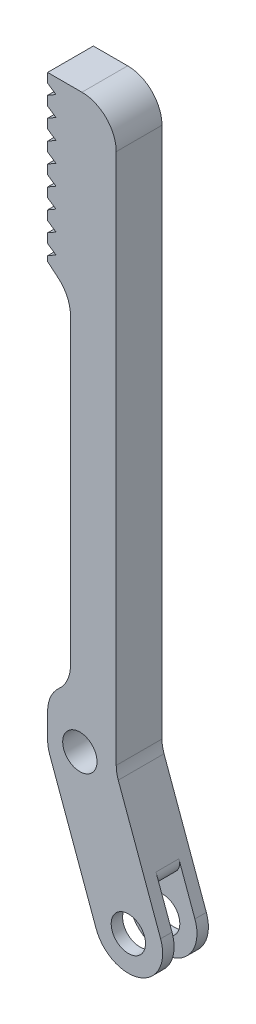
SolidWorks part; units mm, degrees
ref_plane "Front Plane" through (0, 0, 0) normal (0, 0, 1) x (1, 0, 0)
ref_plane "Top Plane" through (0, 0, 0) normal (0, 1, 0) x (1, 0, 0)
ref_plane "Right Plane" through (0, 0, 0) normal (1, 0, 0) x (0, 0, -1)
ref_plane "Plane1" through (0, 0, 20) normal (0, 0, 1) x (1, 0, 0)
sketch "Sketch1" plane through (0, 0, 20) normal (0, 0, 1) x (1, 0, 0)
  line L0 (-35.6011, 326.0365) -> (-35.6011, 70.7467)
  line L1 (-35.6011, 70.7467) -> (-14.3958, 12.4858)
  line L2 (13.7949, 22.7464) -> (-5.6011, 76.0365)
  line L3 (-5.6011, 76.0365) -> (-5.6011, 326.0365)
  line L4 (-5.6011, 326.0365) -> (-35.6011, 326.0365)
  arc A0 (-14.3958, 12.4858) -> (13.7949, 22.7464) centre (-0.3005, 17.6161) ccw
  dimension "D1" = 15
  dimension "D2" = 21.2052
  dimension "D3" = 30
  dimension "D4" = 35.3006
  dimension "D5" = 49.396
  dimension "D6" = 250
extrude "Boss-Extrude1" add sketch "Sketch1" against normal blind 20
sketch "Sketch2" plane through (19.4918, 7.0944, 0) normal (0.9397, 0.342, 0) x (0, 0, -1)
  line L0 (-15, -0.957) -> (-5, -0.957)
  line L1 (-5, -0.957) -> (-5, 32.1615)
  line L2 (-5, 32.1615) -> (-15, 32.1615)
  line L3 (-15, 32.1615) -> (-15, -0.957)
  dimension "D1" = 5
  dimension "D2" = 15
extrude "Cut-Extrude1" cut sketch "Sketch2" against normal up to next
sketch "Sketch3" plane through (0, 0, 0) normal (0, 0, -1) x (-1, 0, 0)
  line L0 (35.6011, 84.1696) -> (35.6011, 254.4275)
  line L1 (35.6011, 254.4275) -> (25.6011, 246.0365)
  line L2 (25.6011, 246.0365) -> (25.6011, 106.5303)
  line L3 (5.6011, 76.0365) -> (5.6011, 326.0365) construction
  line L4 (5.6011, 326.0365) -> (35.6011, 326.0365) construction
  arc A0 (25.6011, 106.5303) -> (30.6011, 95.3499) centre (40.6011, 106.5303) ccw
  arc A1 (30.6011, 95.3499) -> (35.6011, 84.1696) centre (20.6011, 84.1696) cw
  dimension "D1" = 15
  dimension "D2" = 15
  dimension "D3" = 15
  dimension "D4" = 20
  dimension "D5" = 71.609
  dimension "D6" = 80
  dimension "D7" = 219.5063
extrude "Cut-Extrude2" cut sketch "Sketch3" against normal through all
hole_wizard "Ø15.0 (15) Diameter Hole1" positions "Sketch5" profile "Sketch4" hole size "Ø15.0" standard "ANSI Metric"
sketch "Sketch5" plane through (0, 0, 5) normal (0, 0, 1) x (1, 0, 0)
  point P0 (-0.3005, 17.6161)
sketch "Sketch4" plane through (-0.3005, 17.6161, 5) normal (1, 0, 0) x (0, -1, 0)
  line L0 (0, 0) -> (0, 5)
  line L1 (0, 5) -> (7.5, 5)
  line L2 (7.5, 5) -> (7.5, 0)
  line L5 (7.5, 0) -> (0, 0)
  line L11 (0, -6.35) -> (0, 107.95) construction
  dimension "通孔孔直径" = 15
  dimension "通孔孔深度" = 5
hole_wizard "Ø15.0 (15) Diameter Hole2" positions "Sketch7" profile "Sketch6" hole size "Ø15.0" standard "ANSI Metric"
sketch "Sketch7" plane through (0, 0, 0) normal (0, 0, -1) x (-1, 0, 0)
  point P0 (21.5057, 75.877)
sketch "Sketch6" plane through (-21.5057, 75.877, 0) normal (1, 0, 0) x (0, 1, 0)
  line L0 (0, 0) -> (0, 20)
  line L1 (0, 20) -> (7.5, 20)
  line L2 (7.5, 20) -> (7.5, 0)
  line L5 (7.5, 0) -> (0, 0)
  line L11 (0, -6.35) -> (0, 107.95) construction
  dimension "通孔孔直径" = 15
  dimension "通孔孔深度" = 20
hole_wizard "Ø15.0 (15) Diameter Hole3" positions "Sketch9" profile "Sketch8" hole size "Ø15.0" standard "ANSI Metric"
sketch "Sketch9" plane through (0, 0, 15) normal (0, 0, -1) x (-1, 0, 0)
  point P0 (0.3005, 17.6161)
sketch "Sketch8" plane through (-0.3005, 17.6161, 15) normal (1, 0, 0) x (0, 1, 0)
  line L0 (0, 0) -> (0, 5)
  line L1 (0, 5) -> (7.5, 5)
  line L2 (7.5, 5) -> (7.5, 0)
  line L5 (7.5, 0) -> (0, 0)
  line L11 (0, -6.35) -> (0, 107.95) construction
  dimension "通孔孔直径" = 15
  dimension "通孔孔深度" = 5
fillet "Fillet1" radius 5 1 edges at (8.4919, 37.3164, 10)
fillet "Fillet2" radius 15 4 edges at (-35.6011, 70.7467, 10) (-25.6011, 246.0365, 10) (-5.6011, 326.0365, 10) (-5.6011, 76.0365, 10)
sketch "Sketch10" plane through (0, 0, 20) normal (0, 0, 1) x (1, 0, 0)
  line L0 (-35.6011, 321.9744) -> (-31.946, 319.488)
  line L1 (-35.6011, 326.0365) -> (-35.6011, 254.4275) construction
  line L2 (-31.946, 319.488) -> (-35.6011, 317.3625)
  line L3 (-35.6011, 321.9744) -> (-35.6011, 326.0365)
  line L4 (-31.946, 310.814) -> (-35.6011, 308.6885)
  line L5 (-35.6011, 313.3004) -> (-35.6011, 317.3625)
  line L6 (-35.6011, 313.3004) -> (-31.946, 310.814)
  line L7 (-31.946, 302.1399) -> (-35.6011, 300.0145)
  line L8 (-35.6011, 304.6264) -> (-31.946, 302.1399)
  line L9 (-35.6011, 304.6264) -> (-35.6011, 308.6885)
  line L10 (-31.946, 293.4659) -> (-35.6011, 291.3405)
  line L11 (-35.6011, 295.9524) -> (-31.946, 293.4659)
  line L12 (-35.6011, 295.9524) -> (-35.6011, 300.0145)
  line L13 (-31.946, 284.7919) -> (-35.6011, 282.6665)
  line L14 (-35.6011, 287.2784) -> (-31.946, 284.7919)
  line L15 (-35.6011, 287.2784) -> (-35.6011, 291.3405)
  line L16 (-31.946, 276.1179) -> (-35.6011, 273.9924)
  line L17 (-35.6011, 278.6044) -> (-31.946, 276.1179)
  line L18 (-35.6011, 278.6044) -> (-35.6011, 282.6665)
  line L19 (-31.946, 267.4439) -> (-35.6011, 265.3184)
  line L20 (-35.6011, 269.9304) -> (-31.946, 267.4439)
  line L21 (-35.6011, 269.9304) -> (-35.6011, 273.9924)
  line L22 (-31.946, 258.7699) -> (-35.6011, 256.6444)
  line L23 (-35.6011, 261.2564) -> (-31.946, 258.7699)
  line L24 (-35.6011, 261.2564) -> (-35.6011, 265.3184)
  line L25 (-35.6011, 326.0365) -> (-41.3586, 326.0365)
  line L26 (-41.3586, 326.0365) -> (-41.3586, 256.6444)
  line L27 (-41.3586, 256.6444) -> (-35.6011, 256.6444)
  line M12 (-35.6011, 326.0365) -> (-35.6011, 254.4275)
extrude "Cut-Extrude3" cut sketch "Sketch10" against normal blind 20 contours L26 L27 L25 M12 | L6 L4 M12 | L2 L0 M12 | L8 L7 M12 | L11 L10 M12 | L14 L13 M12 | L17 L16 M12 | L20 L19 M12 | L23 L22 M12
scale "Scale1" scale about origin uniform scaling yes scale factor 0.3
